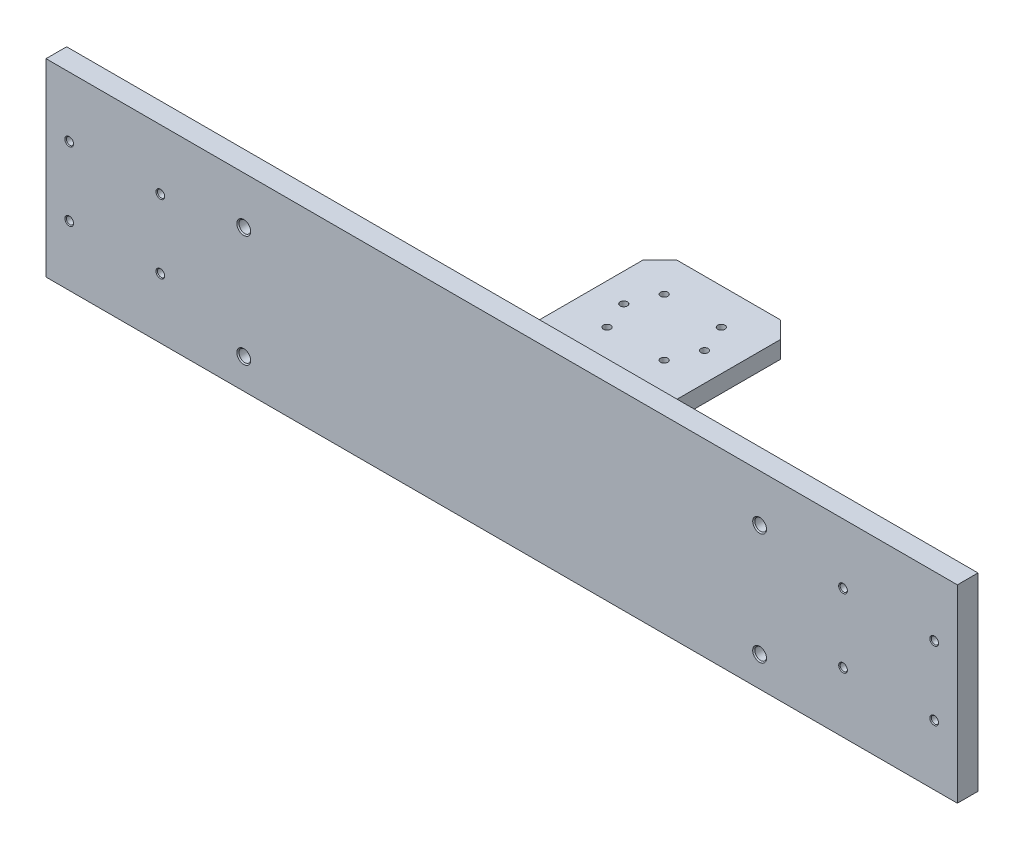
SolidWorks part; units mm, degrees
ref_plane "Front Plane" through (0, 0, 0) normal (0, 0, 1) x (1, 0, 0)
ref_plane "Top Plane" through (0, 0, 0) normal (0, 1, 0) x (1, 0, 0)
ref_plane "Right Plane" through (0, 0, 0) normal (1, 0, 0) x (0, 0, -1)
other "Configuration Table"
sketch "Sketch1" plane through (0, 0, 0) normal (0, 1, 0) x (1, 0, 0)
  line L1 (-50, -98.9671) -> (30, -98.9671)
  line L2 (-50, -98.9671) -> (-50, 21.0329)
  line L3 (-50, 21.0329) -> (30, 21.0329)
  line L4 (30, -98.9671) -> (30, 21.0329)
  line L5 (-50, -98.9671) -> (30, 21.0329) construction
  line L6 (-50, 21.0329) -> (30, -98.9671) construction
  point P0 (-10, -38.9671)
  dimension "D1" = 80
  dimension "D2" = 120
extrude "Boss-Extrude1" add sketch "Sketch1" along normal blind 10
sketch "Sketch2" plane through (0, 0, 98.9671) normal (0, 0, 1) x (1, 0, 0)
  line L0 (-10, 0) -> (-10, 10) construction
  line L1 (-50, 10) -> (30, 10) construction
  line L2 (-50, 0) -> (30, 0) construction
  line L3 (-275, -50) -> (255, -50)
  line L4 (-275, -50) -> (-275, 60)
  line L5 (-275, 60) -> (255, 60)
  line L6 (255, -50) -> (255, 60)
  line L7 (-275, -50) -> (255, 60) construction
  line L8 (-275, 60) -> (255, -50) construction
  point P5 (-10, 5)
  dimension "D1" = 110
  dimension "D2" = 530
extrude "Boss-Extrude2" add sketch "Sketch2" along normal blind 12
chamfer "Chamfer1" distance 10 angle 45 2 edges at (30, 5, -21.0329) (-50, 5, -21.0329)
sketch "Sketch3" plane through (0, 10, 0) normal (0, 1, 0) x (1, 0, 0)
  circle A0 centre (6.617, 0.1499) radius 2.1
  circle A1 centre (13.5, -16.4671) radius 2.1
  circle A2 centre (6.617, -33.0841) radius 2.1
  circle A3 centre (-26.617, -33.0841) radius 2.1
  circle A4 centre (-33.5, -16.4671) radius 2.1
  circle A5 centre (-26.617, 0.1499) radius 2.1
  dimension "D1" = 4.2
extrude "Cut-Extrude1" cut sketch "Sketch3" against normal through all both and the other way through all
hole_wizard "M5 Tapped Hole1" positions "Sketch6" profile "Sketch5" tap size "M5" standard "GB"
sketch "Sketch6" plane through (0, 0, 110.9671) normal (0, 0, 1) x (1, 0, 0)
  line L1 (-275, 5) -> (-180.7063, 5) construction
  line L2 (-275, 60) -> (-275, -50) construction
  line L7 (-10, 60) -> (-10, -50) construction
  line L8 (255, 60) -> (-275, 60) construction
  line L9 (-275, -50) -> (255, -50) construction
  line L11 (255, 5) -> (160.7063, 5) construction
  point P0 (-261.5, 25)
  point P2 (-261.5, -15)
  point P4 (-208.5, 25)
  point P6 (-208.5, -15)
  point P37 (188.5, -15)
  point P38 (188.5, 25)
  point P39 (241.5, -15)
  point P40 (241.5, 25)
  dimension "D1" = 40
  dimension "D2" = 53
  dimension "D3" = 20
  dimension "D4" = 13.5
sketch "Sketch5" plane through (-261.5, 25, 110.9671) normal (1, 0, 0) x (0, -1, 0)
  line L0 (0, 0) -> (0, 13.6618)
  line L1 (0, 13.6618) -> (2.1, 12.4)
  line L2 (2.1, 12.4) -> (2.1, 0.425)
  line L3 (2.1, 0.425) -> (2.525, 0)
  line L5 (2.525, 0) -> (0, 0)
  line L6 (-2.1, 0.425) -> (-2.525, 0) construction
  line L10 (0, 13.6618) -> (-2.1, 12.4) construction
  line L11 (0, -6.35) -> (0, 107.95) construction
  dimension "螺纹孔钻头直径" = 4.2
  dimension "螺纹孔钻头深度" = 12.4
  dimension "近端锥形沉头孔直径" = 5.05
  dimension "近端锥形沉头孔角度" = 90
  dimension "导头角度" = 118
cosmetic thread "Hole Thread Line1" parameters "D1"=10, "D2"=5
cosmetic thread "Hole Thread Line2" parameters "D1"=10, "D2"=5
cosmetic thread "Hole Thread Line3" parameters "D1"=10, "D2"=5
cosmetic thread "Hole Thread Line4" parameters "D1"=10, "D2"=5
cosmetic thread "Hole Thread Line5" parameters "D1"=10, "D2"=5
cosmetic thread "Hole Thread Line6" parameters "D1"=10, "D2"=5
cosmetic thread "Hole Thread Line7" parameters "D1"=10, "D2"=5
cosmetic thread "Hole Thread Line8" parameters "D1"=10, "D2"=5
hole_wizard "M8 Tapped Hole1" positions "Sketch12" profile "Sketch11" tap size "M8" standard "GB"
sketch "Sketch12" plane through (0, 0, 110.9671) normal (0, 0, 1) x (1, 0, 0)
  line L0 (-275, 60) -> (-275, -50) construction
  point P0 (-160, 32.5)
  point P2 (-160, -32.5)
  point P4 (140, 32.5)
  point P6 (140, -32.5)
  dimension "D1" = 300
  dimension "D2" = 65
  dimension "D3" = 115
  dimension "D4" = 32.5
cosmetic thread "Hole Thread Line9" parameters "D1"=16, "D2"=8
cosmetic thread "Hole Thread Line10" parameters "D1"=16, "D2"=8
cosmetic thread "Hole Thread Line11" parameters "D1"=16, "D2"=8
cosmetic thread "Hole Thread Line12" parameters "D1"=16, "D2"=8
sketch "Sketch11" plane through (-160, 32.5, 110.9671) normal (1, 0, 0) x (0, -1, 0)
  line L0 (0, 0) -> (0, 24.2929)
  line L1 (0, 24.2929) -> (3.4, 22.25)
  line L2 (3.4, 22.25) -> (3.4, 0.625)
  line L3 (3.4, 0.625) -> (4.025, 0)
  line L5 (4.025, 0) -> (0, 0)
  line L6 (-3.4, 0.625) -> (-4.025, 0) construction
  line L10 (0, 24.2929) -> (-3.4, 22.25) construction
  line L11 (0, -6.35) -> (0, 107.95) construction
  dimension "螺纹孔钻头直径" = 6.8
  dimension "螺纹孔钻头深度" = 22.25
  dimension "近端锥形沉头孔直径" = 8.05
  dimension "近端锥形沉头孔角度" = 90
  dimension "导头角度" = 118
